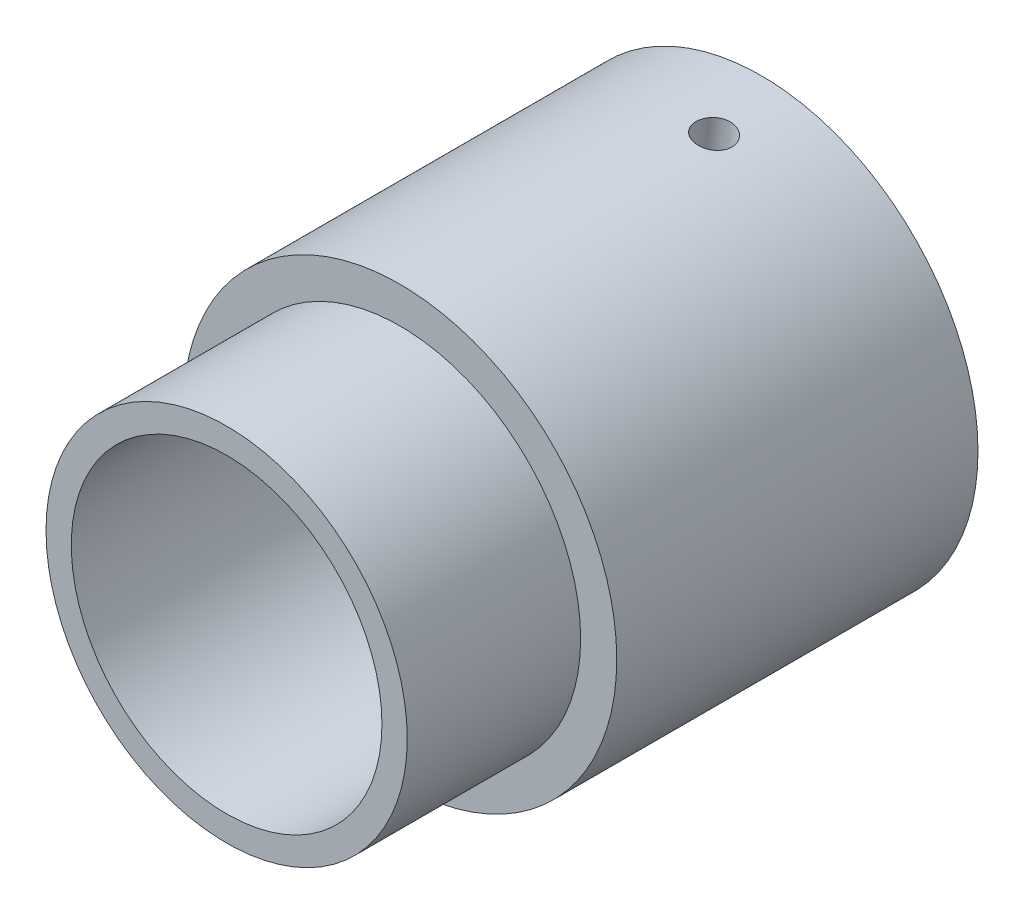
SolidWorks part; units mm, degrees
material "普通碳钢"
ref_plane "Front Plane" through (0, 0, 0) normal (0, 0, 1) x (1, 0, 0)
ref_plane "Top Plane" through (0, 0, 0) normal (0, 1, 0) x (1, 0, 0)
ref_plane "Right Plane" through (0, 0, 0) normal (1, 0, 0) x (0, 0, -1)
sketch "Sketch1" plane through (0, 0, 0) normal (0, 0, 1) x (1, 0, 0)
  circle A0 centre (0, 0) radius 30
  circle A1 centre (0, 0) radius 21.5
  dimension "D1" = 43
  dimension "D2" = 60
extrude "Boss-Extrude1" add sketch "Sketch1" against normal blind 50
hole_wizard "M6 Tapped Hole1" positions "3DSketch2" profile "Sketch3" tap size "M6" standard "GB"
sketch3d "3DSketch2"
  point P0 (3.4711, 29.7985, -40)
  dimension "D1" = 10
sketch "Sketch3" plane through (3.4711, 29.7985, -40) normal (0, 0, 1) x (-0.9933, 0.1157, 0)
  line L0 (0, 0) -> (0, 19.5022)
  line L1 (0, 19.5022) -> (2.5, 18)
  line L2 (2.5, 18) -> (2.5, 0)
  line L5 (2.5, 0) -> (0, 0)
  line L10 (0, 19.5022) -> (-2.5, 18) construction
  line L11 (0, -6.35) -> (0, 107.95) construction
  dimension "螺纹孔钻头直径" = 5
  dimension "螺纹孔钻头深度" = 18
  dimension "导头角度" = 118
cosmetic thread "Tapped hole thread 1" parameters "D1"=8.6458, "D2"=6
sketch "Sketch4" plane through (0, 0, 0) normal (0, 0, 1) x (1, 0, 0)
  circle A0 centre (0, 0) radius 21.5
  circle A1 centre (0, 0) radius 25
  dimension "D1" = 43
  dimension "D2" = 50
extrude "Boss-Extrude2" add sketch "Sketch4" along normal blind 24
